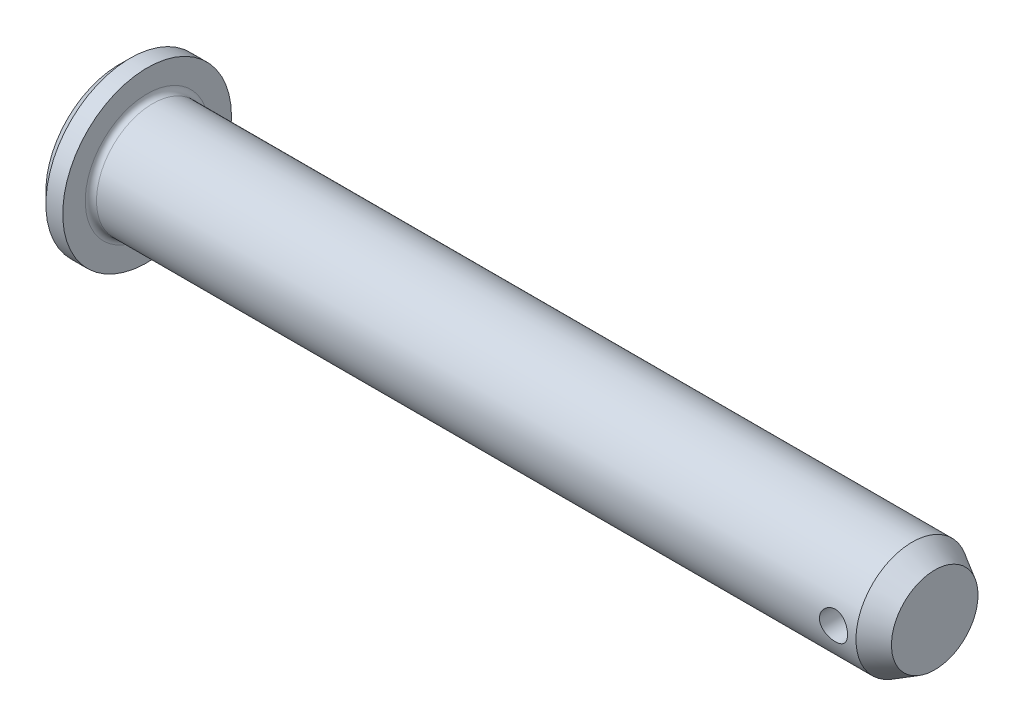
from build123d import *

# Parameters (mm, degrees)
CUT_EXTRUDE1_DEPTH      = 147.543508898
CUT_EXTRUDE1_DEPTH_BACK = 147.543508898
SKETCH2_R               = 2.5
FILLET1_R               = 1
CHAMFER1_SIZE           = 4
CHAMFER1_SIZE2          = 2.309401077


with BuildPart() as part:
    # Sketch1 → Base-Revolve (revolve)
    with BuildSketch(Plane.XY, mode=Mode.PRIVATE) as base_revolve_sk:
        Polygon((0, 0), (145, 0), (145, 10), (5, 10), (5, 15), (2, 15), (0, 13), align=None)
    revolve(base_revolve_sk.sketch.rotate(Axis((0, 0, 0), (-1, 0, 0)), 90), axis=Axis((0, 0, 0), (-1, 0, 0)))

    # Sketch2 → Cut-Extrude1 (cut, two sides: drawn at the far end of the back side and taken through both)
    with BuildSketch(Plane.XY.offset(-CUT_EXTRUDE1_DEPTH_BACK)):
        with Locations((137, 0)):
            Circle(SKETCH2_R)
    extrude(amount=CUT_EXTRUDE1_DEPTH + CUT_EXTRUDE1_DEPTH_BACK, mode=Mode.SUBTRACT)

    # Fillet1
    fillet1_edges = [part.edges().sort_by_distance(p)[0] for p in [
        (5, 0, 10),
    ]]
    fillet(fillet1_edges, radius=FILLET1_R)

    # Chamfer1
    chamfer1_edges = [part.edges().sort_by_distance(p)[0] for p in [
        (145, 0, 10),
    ]]
    chamfer1_side = [part.faces().sort_by_distance(p)[0] for p in [
        (75.5, 0, 10),
    ]]
    chamfer(chamfer1_edges, length=CHAMFER1_SIZE, length2=CHAMFER1_SIZE2, reference=chamfer1_side[0])


solid = part.part
